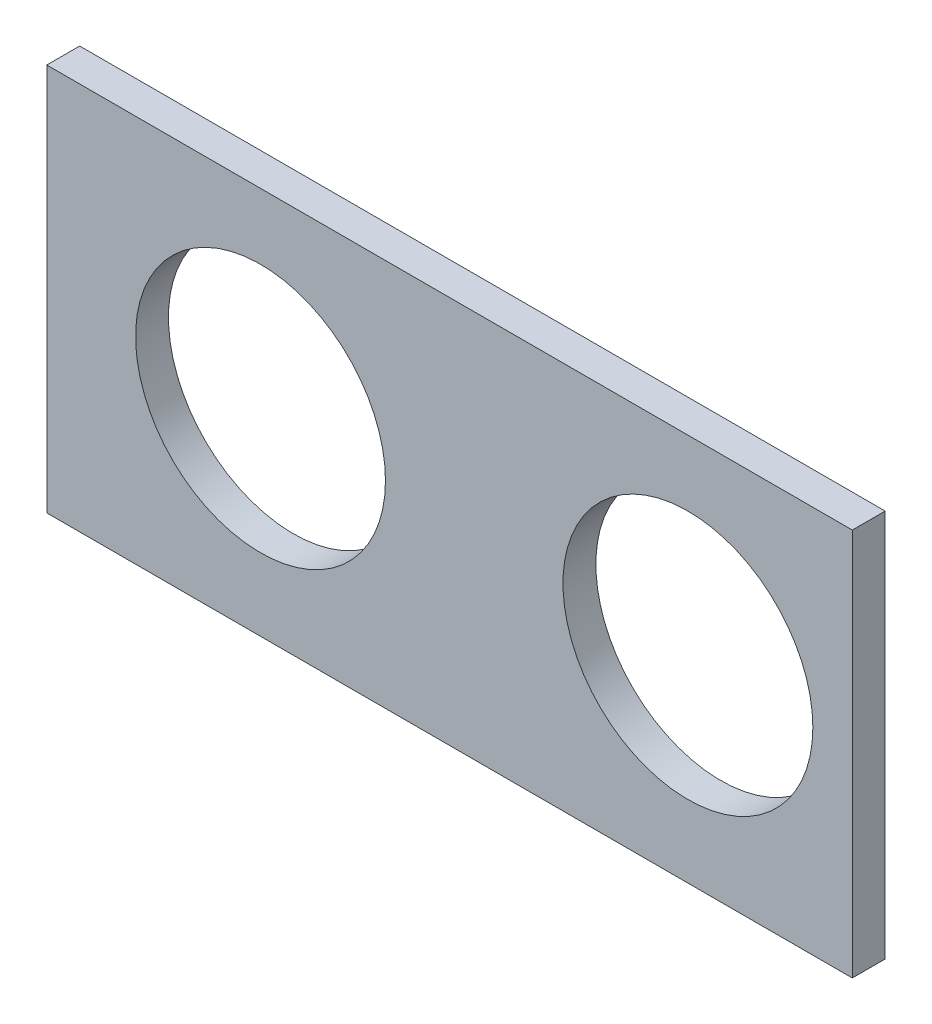
SolidWorks part; units mm, degrees
ref_plane "Front Plane" through (0, 0, 0) normal (0, 0, 1) x (1, 0, 0)
ref_plane "Top Plane" through (0, 0, 0) normal (0, 1, 0) x (1, 0, 0)
ref_plane "Right Plane" through (0, 0, 0) normal (1, 0, 0) x (0, 0, -1)
sketch "Sketch1" plane through (0, 0, 0) normal (0, 0, 1) x (1, 0, 0)
  line L0 (-9.2329, 60) -> (266.8305, 60) construction
  line L1 (0, 0) -> (245, 0)
  line L2 (0, 0) -> (0, 118)
  line L3 (0, 118) -> (245, 118)
  line L4 (245, 0) -> (245, 118)
  line L5 (195, 197.1222) -> (195, -28.1603) construction
  line L6 (65, 178.6564) -> (65, -18.9274) construction
  circle A0 centre (195, 60) radius 38
  circle A1 centre (65, 60) radius 38
  dimension "D6" = 76
  dimension "D7" = 76
  dimension "D1" = 118
  dimension "D2" = 245
  dimension "D3" = 58
  dimension "D4" = 50
  dimension "D5" = 130
extrude "Boss-Extrude1" add sketch "Sketch1" along normal blind 10
